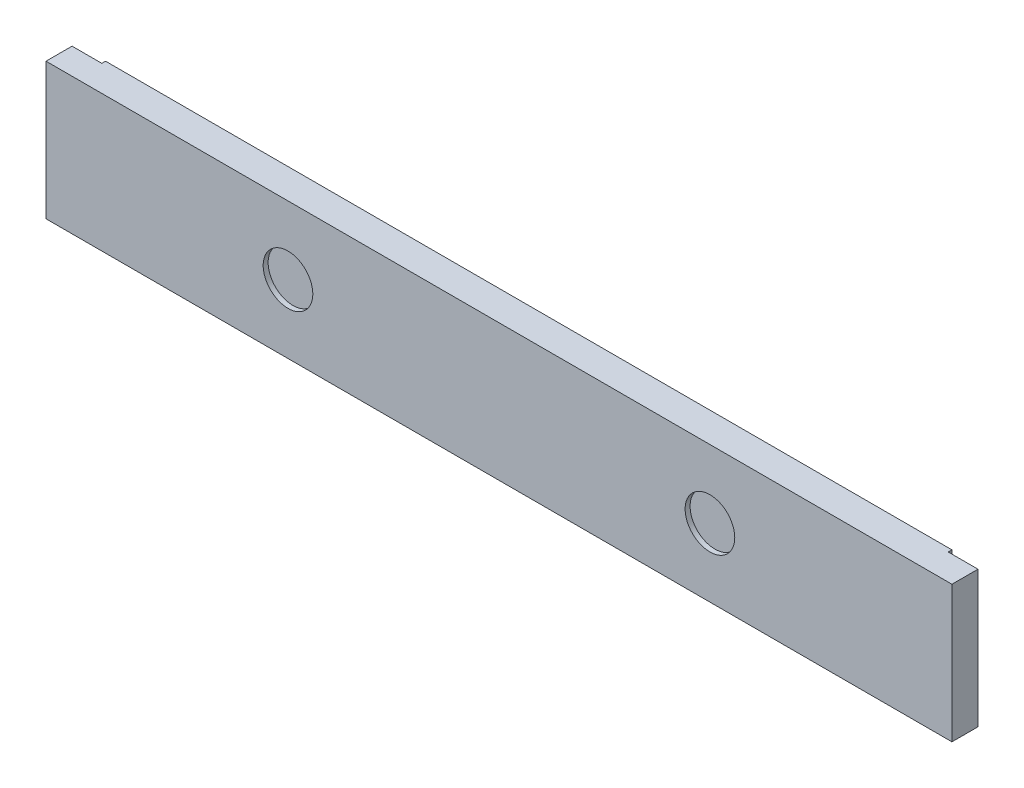
from build123d import *

# Parameters (mm, degrees)
SKETCH_1_W          = 365
SKETCH_1_H          = 55
EXTRUDE_1_DEPTH     = 12
SKETCH_2_R          = 10
CUT_EXTRUDE_1_DEPTH = 2
SKETCH_3_W          = 12
SKETCH_3_H          = 55
CUT_EXTRUDE_2_DEPTH = 1.5


with BuildPart() as part:
    # 草图1 → 凸台-拉伸1 (new body)
    with BuildSketch(Plane.XY):
        Rectangle(SKETCH_1_W, SKETCH_1_H)
    extrude(amount=EXTRUDE_1_DEPTH)

    # 草图2 → 切除-拉伸1 (cut)
    with BuildSketch(Plane.XY.offset(12)):
        with Locations((85, 0)):
            Circle(SKETCH_2_R)
        with Locations((-85, 0)):
            Circle(SKETCH_2_R)
    extrude(amount=-CUT_EXTRUDE_1_DEPTH, mode=Mode.SUBTRACT)

    # 草图3 → 切除-拉伸2 (cut)
    with BuildSketch(Plane(origin=(0, 0, 0), x_dir=(-1, 0, 0), z_dir=(0, 0, -1))):
        with Locations((176.5, 0)):
            Rectangle(SKETCH_3_W, SKETCH_3_H)
        with Locations((-176.5, 0)):
            Rectangle(SKETCH_3_W, SKETCH_3_H)
    extrude(amount=-CUT_EXTRUDE_2_DEPTH, mode=Mode.SUBTRACT)


solid = part.part
